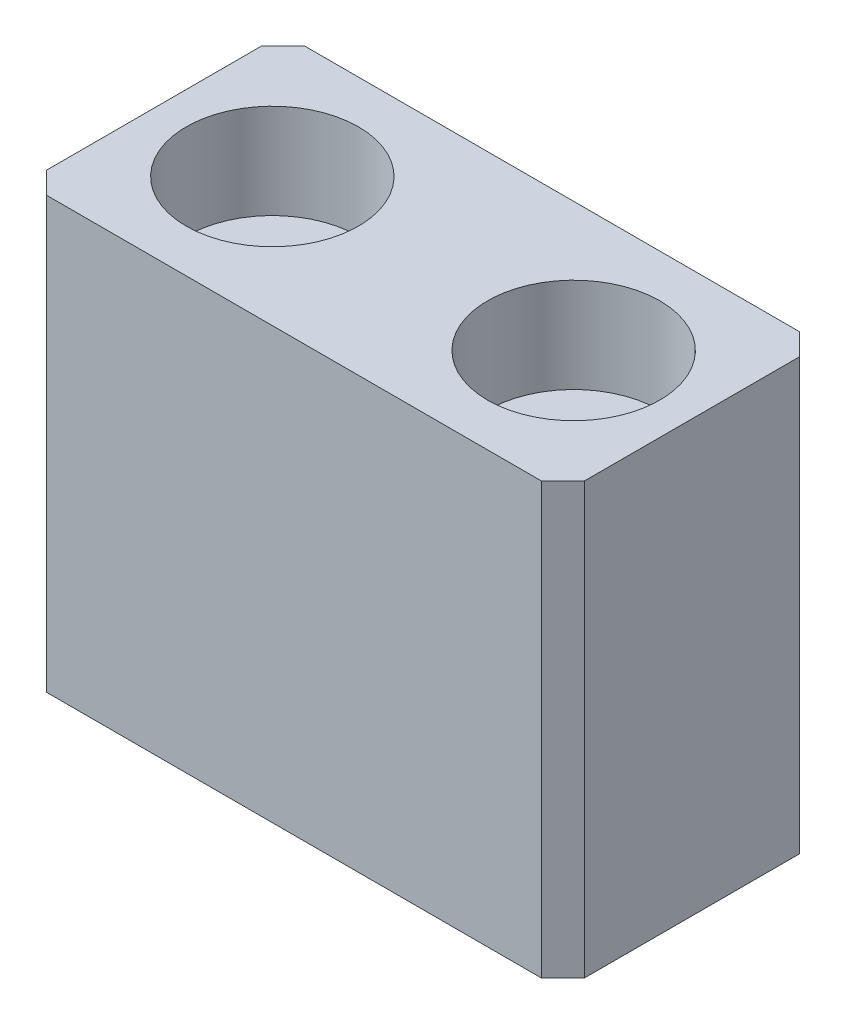
from build123d import *

# Parameters (mm, degrees)
SKETCH1_W                                           = 25
SKETCH1_H                                           = 20
BOSS_EXTRUDE1_DEPTH                                 = 12
CBORE_FOR_M4_HEX_SOCKET_HEAD_CAP_SCREW1_D           = 4.5
CBORE_FOR_M4_HEX_SOCKET_HEAD_CAP_SCREW1_CBORE_D     = 8
CBORE_FOR_M4_HEX_SOCKET_HEAD_CAP_SCREW1_CBORE_DEPTH = 4.4
CHAMFER1_SIZE                                       = 1


with BuildPart() as part:
    # Sketch1 → Boss-Extrude1 (new body)
    with BuildSketch(Plane.XY):
        Rectangle(SKETCH1_W, SKETCH1_H)
    extrude(amount=BOSS_EXTRUDE1_DEPTH)

    # CBORE for M4 Hex Socket Head Cap Screw1 (through all)
    with Locations(Plane(origin=(0, 10, 0), x_dir=(1, 0, 0), z_dir=(0, 1, 0))):
        with Locations((-7, -6), (7, -6)):
            CounterBoreHole(CBORE_FOR_M4_HEX_SOCKET_HEAD_CAP_SCREW1_D / 2, CBORE_FOR_M4_HEX_SOCKET_HEAD_CAP_SCREW1_CBORE_D / 2, CBORE_FOR_M4_HEX_SOCKET_HEAD_CAP_SCREW1_CBORE_DEPTH)

    # Chamfer1
    chamfer1_edges = [part.edges().sort_by_distance(p)[0] for p in [
        (-12.5, 0, 12),
        (12.5, 0, 12),
        (-12.5, 0, 0),
        (12.5, 0, 0),
    ]]
    chamfer(chamfer1_edges, length=CHAMFER1_SIZE)


solid = part.part
